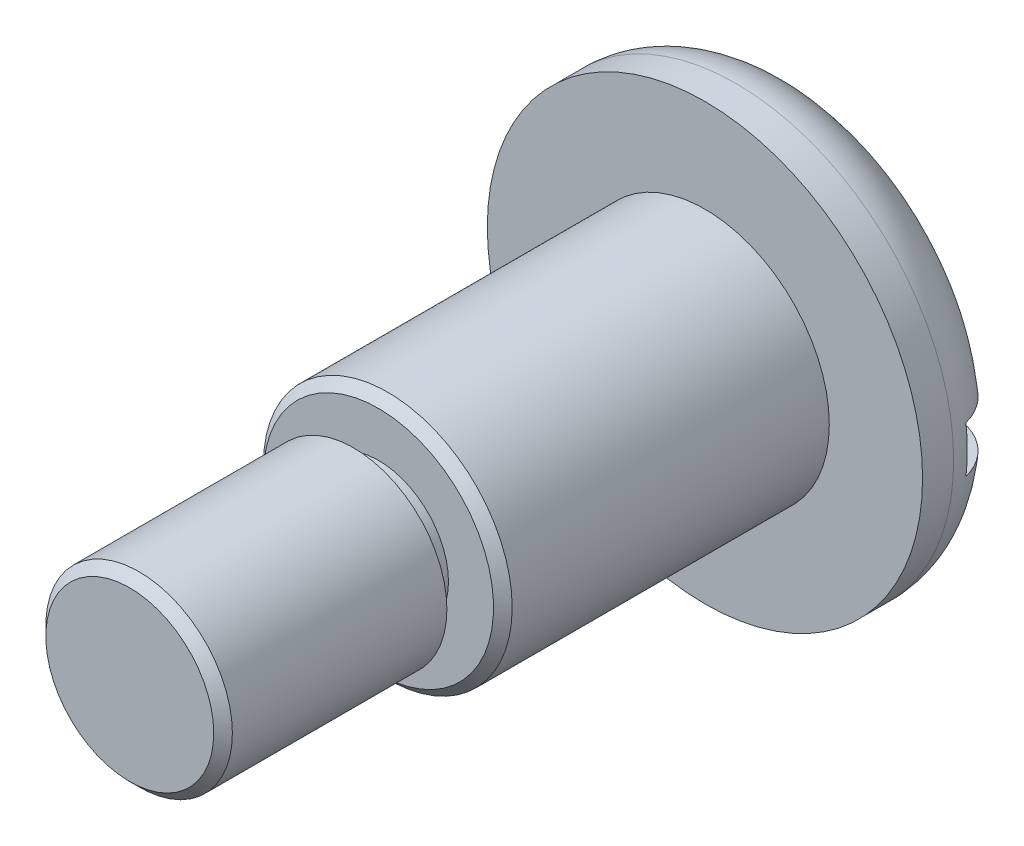
SolidWorks part; units mm, degrees
material "SUS304"
ref_plane "前视基准面" through (0, 0, 0) normal (0, 0, 1) x (1, 0, 0)
ref_plane "上视基准面" through (0, 0, 0) normal (0, 1, 0) x (1, 0, 0)
ref_plane "右视基准面" through (0, 0, 0) normal (1, 0, 0) x (0, 0, -1)
sketch "草图1" plane through (0, 0, 0) normal (0, 0, 1) x (1, 0, 0)
  circle A0 centre (0, 0) radius 7
  dimension "D1" = 14
extrude "凸台-拉伸1" add sketch "草图1" along normal blind 3
sketch "草图2" plane through (0, 0, 3) normal (0, 0, 1) x (1, 0, 0)
  circle A0 centre (0, 0) radius 4
  dimension "D1" = 8
extrude "凸台-拉伸2" add sketch "草图2" along normal blind 10.5
sketch "草图3" plane through (0, 0, 13.5) normal (0, 0, 1) x (1, 0, 0)
  circle A0 centre (0, 0) radius 3
  dimension "D1" = 6
extrude "凸台-拉伸3" add sketch "草图3" along normal blind 8
cosmetic thread "装饰螺纹线1" parameters "D2"=4.917
sketch "草图4" plane through (0, 0, 13.5) normal (0, 0, 1) x (1, 0, 0)
  circle A0 centre (0, 0) radius 3
  circle A1 centre (0, 0) radius 2.25
  circle A2 centre (0, 0) radius 3 construction
  dimension "D1" = 4.5
extrude "切除-拉伸1" cut sketch "草图4" along normal blind 0.8
fillet "圆角1" radius 2 1 edges at (7, 0, 0)
sketch "草图5" plane through (0, 0, 0) normal (0, 0, -1) x (-1, 0, 0)
  line L1 (-8.5177, -0.75) -> (8.5177, -0.75)
  line L2 (-8.5177, -0.75) -> (-8.5177, 0.75)
  line L3 (-8.5177, 0.75) -> (8.5177, 0.75)
  line L4 (8.5177, -0.75) -> (8.5177, 0.75)
  line L5 (-8.5177, -0.75) -> (8.5177, 0.75) construction
  line L6 (-8.5177, 0.75) -> (8.5177, -0.75) construction
  point P0 (0, 0)
  dimension "D1" = 1.5
extrude "切除-拉伸2" cut sketch "草图5" against normal blind 1.5
chamfer "倒角1" distance 0.3 angle 45 2 edges at (4, 0, 13.5) (3, 0, 21.5)
